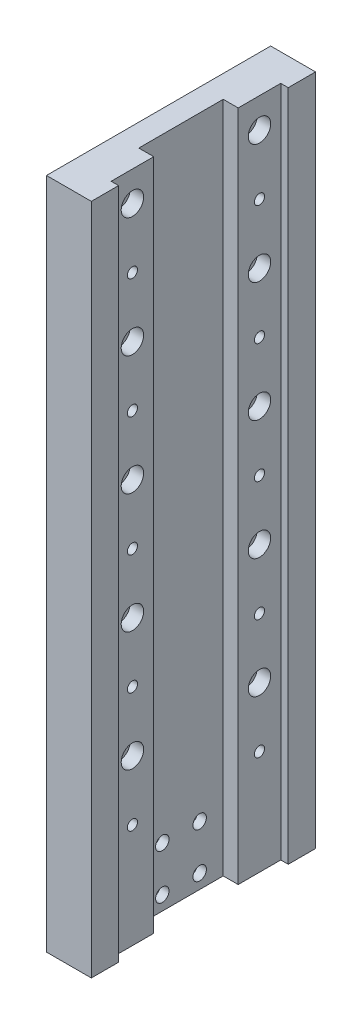
from build123d import *

# Parameters (mm, degrees)
SKETCH_1_W                = 150
SKETCH_1_H                = 450
EXTRUDE_1_DEPTH           = 30
SKETCH_2_W                = 28.5
SKETCH_2_H                = 450
CUT_EXTRUDE_1_DEPTH       = 5
HOLE_WIZARD_M8_1_D        = 6.8
PATTERN_LINEAR_1_COUNT    = 5
PATTERN_LINEAR_1_PITCH    = 80
HOLE_WIZARD_1_D           = 9
HOLE_WIZARD_1_CBORE_D     = 15
HOLE_WIZARD_1_CBORE_DEPTH = 9
PATTERN_LINEAR_2_COUNT    = 5
PATTERN_LINEAR_2_PITCH    = 80
SKETCH_7_W                = 56.5
SKETCH_7_H                = 450
CUT_EXTRUDE_2_DEPTH       = 15
HOLE_WIZARD_2_D           = 9
HOLE_WIZARD_2_CBORE_D     = 15
HOLE_WIZARD_2_CBORE_DEPTH = 9


with BuildPart() as part:
    # 草图1 → 凸台-拉伸1 (new body)
    with BuildSketch(Plane(origin=(0, 0, 0), x_dir=(0, 0, -1), z_dir=(1, 0, 0))):
        Rectangle(SKETCH_1_W, SKETCH_1_H)
    extrude(amount=EXTRUDE_1_DEPTH)

    # 草图2 → 切除-拉伸1 (cut)
    with BuildSketch(Plane(origin=(30, 0, 0), x_dir=(0, 0, -1), z_dir=(1, 0, 0))):
        with Locations((-42.5, 0)):
            Rectangle(SKETCH_2_W, SKETCH_2_H)
        with Locations((42.5, 0)):
            Rectangle(SKETCH_2_W, SKETCH_2_H)
    extrude(amount=-CUT_EXTRUDE_1_DEPTH, mode=Mode.SUBTRACT)

    # M8 螺纹孔1 (through all)
    with Locations(Plane(origin=(30, 0, 0), x_dir=(0, 0, -1), z_dir=(1, 0, 0))):
        with Locations((-42.5, -155), (42.5, -155)):
            hole_wizard_m8_1 = Hole(HOLE_WIZARD_M8_1_D / 2)

    # 阵列(线性)1: M8 螺纹孔1 ×5
    with Locations(*[(0, i * PATTERN_LINEAR_1_PITCH, 0) for i in range(1, PATTERN_LINEAR_1_COUNT)]):
        add(hole_wizard_m8_1, mode=Mode.SUBTRACT)

    # 打孔尺寸(%根据)内六角圆柱头螺钉的类型1 (through all)
    with Locations(Plane(origin=(25, 0, 0), x_dir=(0, 0, -1), z_dir=(1, 0, 0))):
        with Locations((-42.5, -115), (42.5, -115)):
            hole_wizard_1 = CounterBoreHole(HOLE_WIZARD_1_D / 2, HOLE_WIZARD_1_CBORE_D / 2, HOLE_WIZARD_1_CBORE_DEPTH)

    # 阵列(线性)2: 打孔尺寸(%根据)内六角圆柱头螺钉的类型1 ×5
    with Locations(*[(0, i * PATTERN_LINEAR_2_PITCH, 0) for i in range(1, PATTERN_LINEAR_2_COUNT)]):
        add(hole_wizard_1, mode=Mode.SUBTRACT)

    # 草图7 → 切除-拉伸2 (cut)
    with BuildSketch(Plane(origin=(30, 0, 0), x_dir=(0, 0, -1), z_dir=(1, 0, 0))):
        Rectangle(SKETCH_7_W, SKETCH_7_H)
    extrude(amount=-CUT_EXTRUDE_2_DEPTH, mode=Mode.SUBTRACT)

    # 打孔尺寸(%根据)内六角圆柱头螺钉的类型2 (through all)
    with Locations(Plane(origin=(0, 0, 0), x_dir=(0, 0, -1), z_dir=(-1, 0, 0))):
        with Locations((-12.5, 185.5), (12.5, 185.5), (-12.5, 215.5), (12.5, 215.5)):
            CounterBoreHole(HOLE_WIZARD_2_D / 2, HOLE_WIZARD_2_CBORE_D / 2, HOLE_WIZARD_2_CBORE_DEPTH)


solid = part.part
